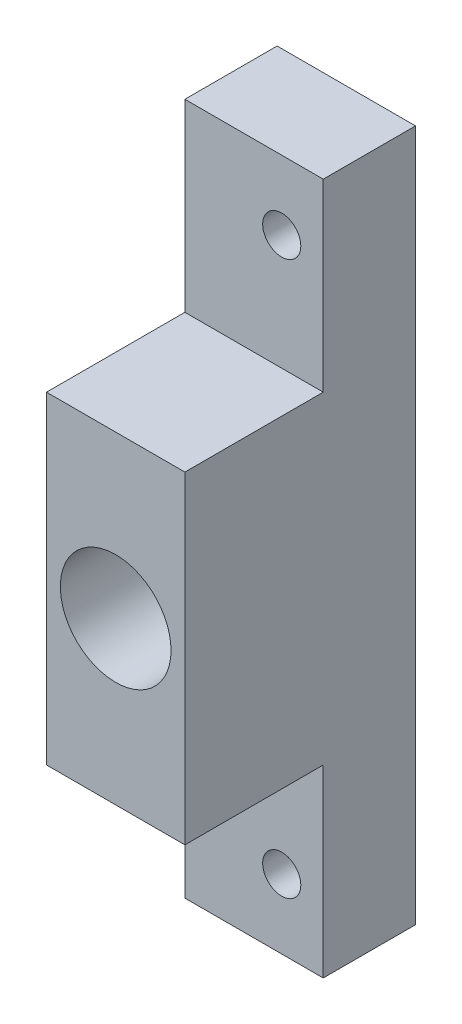
from build123d import *

# Parameters (mm, degrees)
SKETCH1_W           = 15
SKETCH1_H           = 75
BOSS_EXTRUDE1_DEPTH = 25
SKETCH2_R           = 2.067
CUT_EXTRUDE1_DEPTH  = 25
SKETCH3_W           = 15
SKETCH3_H           = 20
CUT_EXTRUDE2_DEPTH  = 15
SKETCH4_R           = 6
CUT_EXTRUDE3_DEPTH  = 20


with BuildPart() as part:
    # Sketch1 → Boss-Extrude1 (new body)
    with BuildSketch(Plane.XY):
        with Locations((-29.5, 0)):
            Rectangle(SKETCH1_W, SKETCH1_H)
    extrude(amount=BOSS_EXTRUDE1_DEPTH)

    # Sketch2 → Cut-Extrude1 (cut)
    with BuildSketch(Plane.XY.offset(25)):
        with Locations((-26.5, 30)):
            Circle(SKETCH2_R)
        with Locations((-26.5, -30)):
            Circle(SKETCH2_R)
    extrude(amount=-CUT_EXTRUDE1_DEPTH, mode=Mode.SUBTRACT)

    # Sketch3 → Cut-Extrude2 (cut)
    with BuildSketch(Plane.XY.offset(25)):
        with Locations((-29.5, 27.5)):
            Rectangle(SKETCH3_W, SKETCH3_H)
        with Locations((-29.5, -27.5)):
            Rectangle(SKETCH3_W, SKETCH3_H)
    extrude(amount=-CUT_EXTRUDE2_DEPTH, mode=Mode.SUBTRACT)

    # Sketch4 → Cut-Extrude3 (cut)
    with BuildSketch(Plane.XY.offset(25)):
        with Locations((-29.5, 0)):
            Circle(SKETCH4_R)
    extrude(amount=-CUT_EXTRUDE3_DEPTH, mode=Mode.SUBTRACT)


solid = part.part
